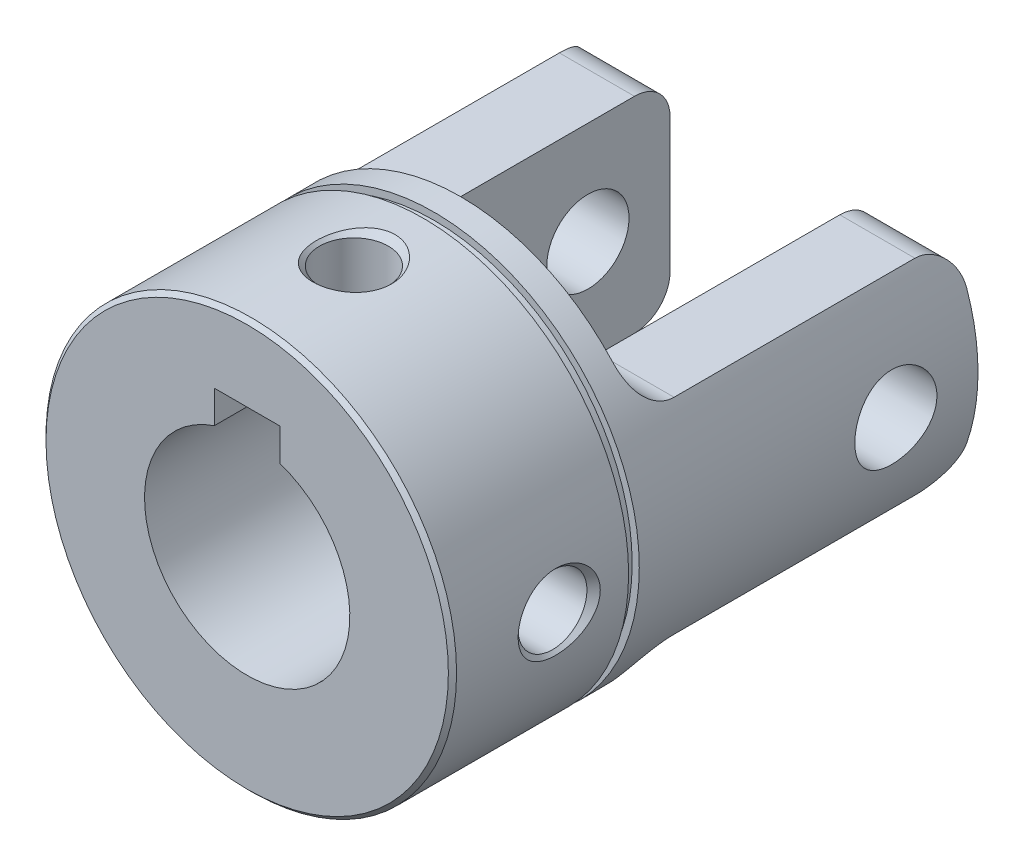
from build123d import *

# Parameters (mm, degrees)
CUT_EXTRUDE_1_DEPTH      = 25
CUT_EXTRUDE_1_DEPTH_BACK = 25
CUT_EXTRUDE_2_DEPTH      = 25
CUT_EXTRUDE_2_DEPTH_BACK = 25
SKETCH_3_W               = 25
SKETCH_3_H               = 38
CUT_EXTRUDE_3_DEPTH      = 25
CUT_EXTRUDE_3_DEPTH_BACK = 25
SKETCH_4_R               = 5
SKETCH_7_W               = 8
SKETCH_7_H               = 15.8
CUT_EXTRUDE_4_DEPTH      = 26


with BuildPart() as part:
    # 草图1 → 旋转1 (revolve)
    with BuildSketch(Plane(origin=(0, 0, 0), x_dir=(0, 0, -1), z_dir=(1, 0, 0)), mode=Mode.PRIVATE) as revolve_1_sk:
        Polygon((26, 0), (26, 12.5), (0, 12.5), (0, 24.5), (0.5, 25), (21.45, 25), (21.45, 24.133333333), (22.75, 24.133333333), (22.75, 25), (64, 25), (64, 0), align=None)
    revolve(revolve_1_sk.sketch.rotate(Axis((0, 0, -64), (0, 0, 1)), 270), axis=Axis((0, 0, -64), (0, 0, 1)))

    # 草图2 → 切除-拉伸1 (cut, two sides: drawn at the far end of the back side and taken through both)
    with BuildSketch(Plane(origin=(0, 0, 0), x_dir=(0, 0, -1), z_dir=(1, 0, 0)).offset(-CUT_EXTRUDE_1_DEPTH_BACK)):
        with BuildLine():
            Line((30.333333333, 12.5), (59.666666667, 12.5))
            ThreePointArc((59.666666667, 12.5), (62.730796052, 11.230796052), (64, 8.166666667))
            Line((64, 8.166666667), (64, -8.166666667))
            ThreePointArc((64, -8.166666667), (62.730796052, -11.230796052), (59.666666667, -12.5))
            Line((59.666666667, -12.5), (30.333333333, -12.5))
            ThreePointArc((30.333333333, -12.5), (27.269203948, -13.769203948), (26, -16.833333333))
            Line((26, -16.833333333), (26, -25))
            Line((26, -25), (69, -25))
            Line((69, -25), (69, 25))
            Line((69, 25), (26, 25))
            Line((26, 25), (26, 16.833333333))
            ThreePointArc((26, 16.833333333), (27.269203948, 13.769203948), (30.333333333, 12.5))
        make_face()
    extrude(amount=CUT_EXTRUDE_1_DEPTH + CUT_EXTRUDE_1_DEPTH_BACK, mode=Mode.SUBTRACT)

    # 草图3 → 切除-拉伸2 (cut, two sides: drawn at the far end of the back side and taken through both)
    with BuildSketch(Plane(origin=(0, 0, 0), x_dir=(1, 0, 0), z_dir=(0, 1, 0)).offset(-CUT_EXTRUDE_2_DEPTH_BACK)):
        with Locations((0, 45)):
            Rectangle(SKETCH_3_W, SKETCH_3_H)
    extrude(amount=CUT_EXTRUDE_2_DEPTH + CUT_EXTRUDE_2_DEPTH_BACK, mode=Mode.SUBTRACT)

    # 草图4 → 切除-拉伸3 (cut, two sides: drawn at the far end of the back side and taken through both)
    with BuildSketch(Plane(origin=(0, 0, 0), x_dir=(0, 0, -1), z_dir=(1, 0, 0)).offset(-CUT_EXTRUDE_3_DEPTH_BACK)):
        with Locations((54, 0)):
            Circle(SKETCH_4_R)
    extrude(amount=CUT_EXTRUDE_3_DEPTH + CUT_EXTRUDE_3_DEPTH_BACK, mode=Mode.SUBTRACT)

    # 草图5 → 切除-旋转1 (revolve, cut)
    with BuildSketch(Plane(origin=(0, 0, 0), x_dir=(0, 0, -1), z_dir=(1, 0, 0)), mode=Mode.PRIVATE) as cut_revolve_1_sk:
        Polygon((13, 25), (18, 25), (17.188, 24.188), (17.188, 0), (13, 0), align=None)
    revolve(cut_revolve_1_sk.sketch.rotate(Axis((0, 0, -13), (0, 1, 0)), 180), axis=Axis((0, 0, -13), (0, 1, 0)), mode=Mode.SUBTRACT)

    # 草图6 → 切除-旋转2 (revolve, cut)
    with BuildSketch(Plane(origin=(0, 0, 0), x_dir=(1, 0, 0), z_dir=(0, 1, 0)), mode=Mode.PRIVATE) as cut_revolve_2_sk:
        Polygon((25, 13), (25, 8), (24.188, 8.812), (0, 8.812), (0, 13), align=None)
    revolve(cut_revolve_2_sk.sketch.rotate(Axis((0, 0, -13), (1, 0, 0)), 180), axis=Axis((0, 0, -13), (1, 0, 0)), mode=Mode.SUBTRACT)

    # 草图7 → 切除-拉伸4 (cut)
    with BuildSketch(Plane.XY):
        with Locations((0, 7.9)):
            Rectangle(SKETCH_7_W, SKETCH_7_H)
    extrude(amount=-CUT_EXTRUDE_4_DEPTH, mode=Mode.SUBTRACT)


solid = part.part
